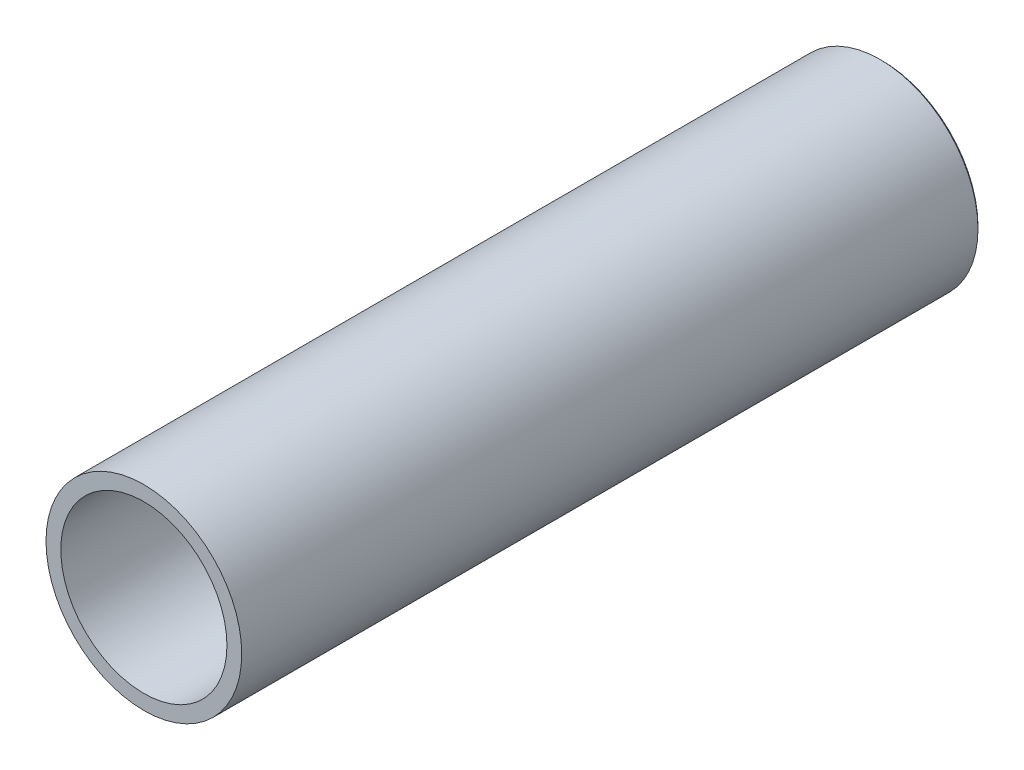
SolidWorks part; units mm, degrees
material "1023 碳钢板 (SS)"
ref_plane "前视基准面" through (0, 0, 0) normal (0, 0, 1) x (1, 0, 0)
ref_plane "上视基准面" through (0, 0, 0) normal (0, 1, 0) x (1, 0, 0)
ref_plane "右视基准面" through (0, 0, 0) normal (1, 0, 0) x (0, 0, -1)
sketch "草图1" plane through (0, 0, 0) normal (0, 0, 1) x (1, 0, 0)
  circle A0 centre (0, 0) radius 21.2
  dimension "D1" = 42.4
extrude "凸台-拉伸1" add sketch "草图1" along normal blind 160
shell "抽壳1" thickness 3.2
chamfer "倒角1" distance 0.5 angle 45 1 edges at (21.2, 0, 0)
